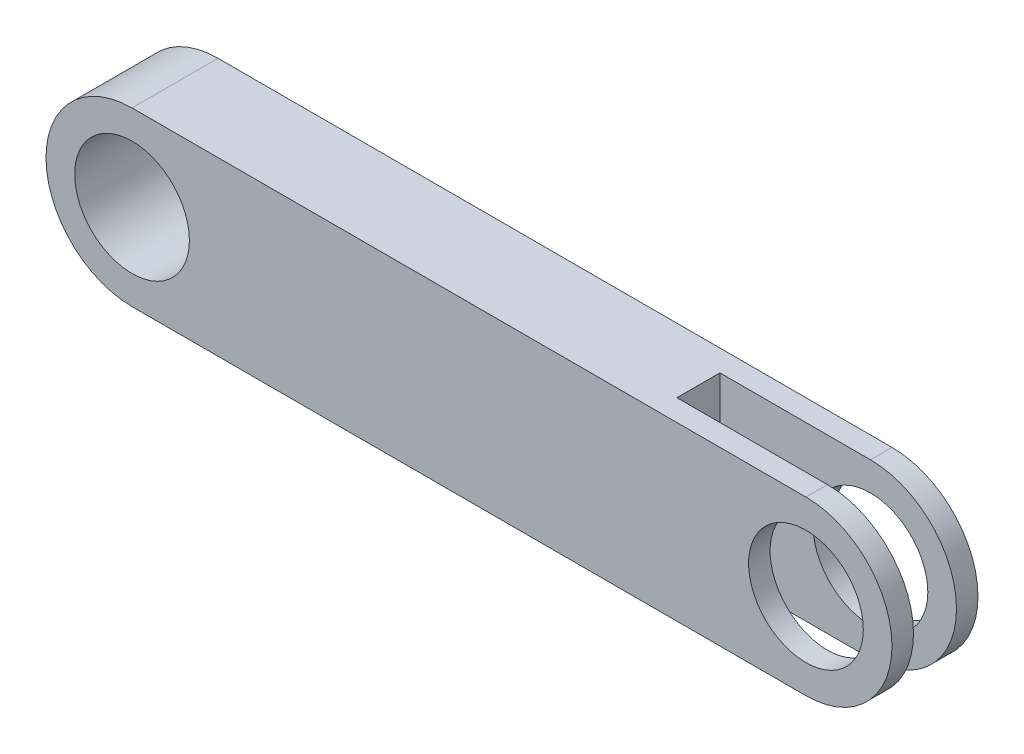
SolidWorks part; units mm, degrees
ref_plane "Front Plane" through (0, 0, 0) normal (0, 0, 1) x (1, 0, 0)
ref_plane "Top Plane" through (0, 0, 0) normal (0, 1, 0) x (1, 0, 0)
ref_plane "Right Plane" through (0, 0, 0) normal (1, 0, 0) x (0, 0, -1)
other "Configuration Table"
sketch "Sketch1" plane through (0, 0, 0) normal (0, 0, 1) x (1, 0, 0)
  line L0 (23.5, 0) -> (-23.5, 0) construction
  line L1 (23.5, -6) -> (-23.5, -6)
  line L2 (23.5, 6) -> (-23.5, 6)
  arc A0 (23.5, -6) -> (23.5, 6) centre (23.5, 0) ccw
  arc A1 (-23.5, 6) -> (-23.5, -6) centre (-23.5, 0) ccw
  point P2 (0, 0)
  dimension "D2" = 6
  dimension "D1" = 47
extrude "Boss-Extrude1" add sketch "Sketch1" along normal blind 6
sketch "Sketch2" plane through (0, 6, 0) normal (0, 1, 0) x (1, 0, 0)
  line L0 (29.5, -6) -> (29.5, 0) construction
  line L1 (13, -1.5) -> (46, -1.5)
  line L2 (13, -1.5) -> (13, -4.5)
  line L3 (13, -4.5) -> (46, -4.5)
  line L4 (46, -1.5) -> (46, -4.5)
  line L5 (13, -1.5) -> (46, -4.5) construction
  line L6 (13, -4.5) -> (46, -1.5) construction
  line L7 (23.5, -6) -> (23.5, 0) construction
  point P0 (29.5, -3)
  dimension "D1" = 3
  dimension "D2" = 10.5
extrude "Cut-Extrude1" cut sketch "Sketch2" against normal blind 35
sketch "Sketch3" plane through (0, 0, 6) normal (0, 0, 1) x (1, 0, 0)
  circle A0 centre (23.5, 0) radius 4
  circle A1 centre (-23.5, 0) radius 4
  dimension "D1" = 8
extrude "Cut-Extrude2" cut sketch "Sketch3" against normal blind 35
